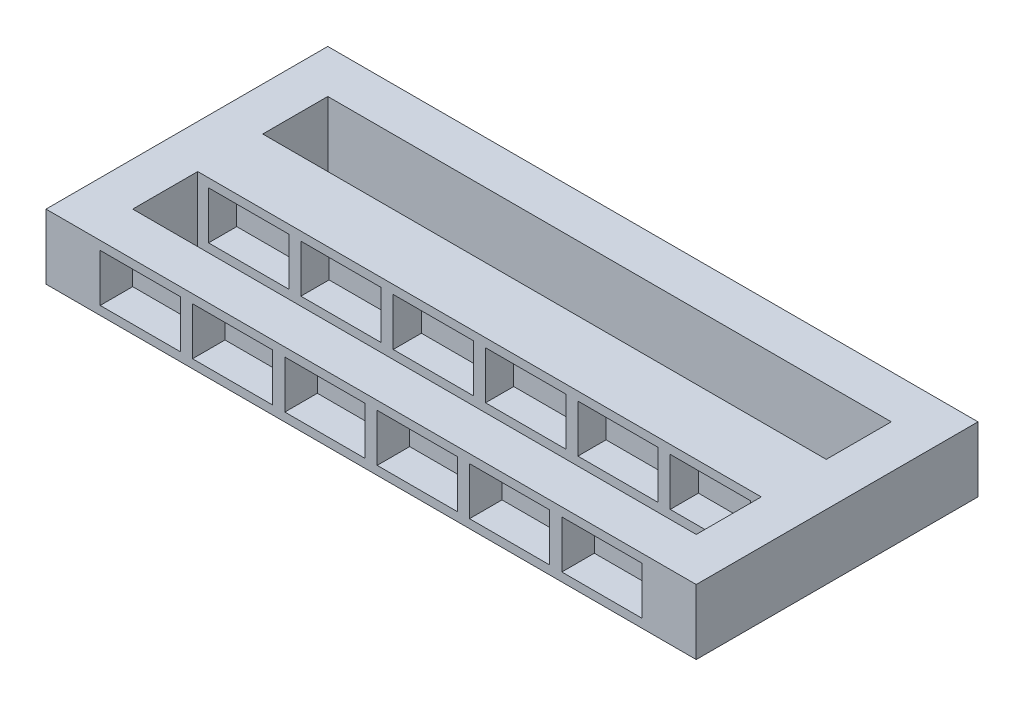
from build123d import *

# Parameters (mm, degrees)
SKETCH1_W           = 3000
SKETCH1_H           = 1300
SKETCH1_W_2         = 2600
SKETCH1_H_2         = 300
BOSS_EXTRUDE1_DEPTH = 300
SKETCH2_W           = 370
SKETCH2_H           = 220
CUT_EXTRUDE1_DEPTH  = 150
SKETCH3_W           = 370
SKETCH3_H           = 220
CUT_EXTRUDE2_DEPTH  = 130


with BuildPart() as part:
    # Sketch1 → Boss-Extrude1 (new body)
    with BuildSketch(Plane(origin=(0, 0, 0), x_dir=(1, 0, 0), z_dir=(0, 1, 0))):
        Rectangle(SKETCH1_W, SKETCH1_H)
        with Locations((0, 300)):
            Rectangle(SKETCH1_W_2, SKETCH1_H_2, mode=Mode.SUBTRACT)
        with Locations((0, -300)):
            Rectangle(SKETCH1_W_2, SKETCH1_H_2, mode=Mode.SUBTRACT)
    extrude(amount=BOSS_EXTRUDE1_DEPTH)

    # Sketch2 → Cut-Extrude1 (cut)
    with BuildSketch(Plane.XY.offset(650)):
        with Locations((-1065, 150)):
            Rectangle(SKETCH2_W, SKETCH2_H)
        with Locations((1065, 150)):
            Rectangle(SKETCH2_W, SKETCH2_H)
        with Locations((-639, 150)):
            Rectangle(SKETCH2_W, SKETCH2_H)
        with Locations((-213, 150)):
            Rectangle(SKETCH2_W, SKETCH2_H)
        with Locations((213, 150)):
            Rectangle(SKETCH2_W, SKETCH2_H)
        with Locations((639, 150)):
            Rectangle(SKETCH2_W, SKETCH2_H)
    cut_extrude1 = extrude(amount=-CUT_EXTRUDE1_DEPTH, mode=Mode.SUBTRACT)

    # Mirror1: Cut-Extrude1 across plane
    add(cut_extrude1.mirror(Plane.XY), mode=Mode.SUBTRACT)

    # Sketch3 → Cut-Extrude2 (cut)
    with BuildSketch(Plane.XY.offset(150)):
        with Locations((-1065, 150)):
            Rectangle(SKETCH3_W, SKETCH3_H)
        with Locations((-639, 150)):
            Rectangle(SKETCH3_W, SKETCH3_H)
        with Locations((-213, 150)):
            Rectangle(SKETCH3_W, SKETCH3_H)
        with Locations((213, 150)):
            Rectangle(SKETCH3_W, SKETCH3_H)
        with Locations((639, 150)):
            Rectangle(SKETCH3_W, SKETCH3_H)
        with Locations((1065, 150)):
            Rectangle(SKETCH3_W, SKETCH3_H)
    cut_extrude2 = extrude(amount=-CUT_EXTRUDE2_DEPTH, mode=Mode.SUBTRACT)

    # Mirror2: Cut-Extrude2 across plane
    add(cut_extrude2.mirror(Plane.XY), mode=Mode.SUBTRACT)


solid = part.part
